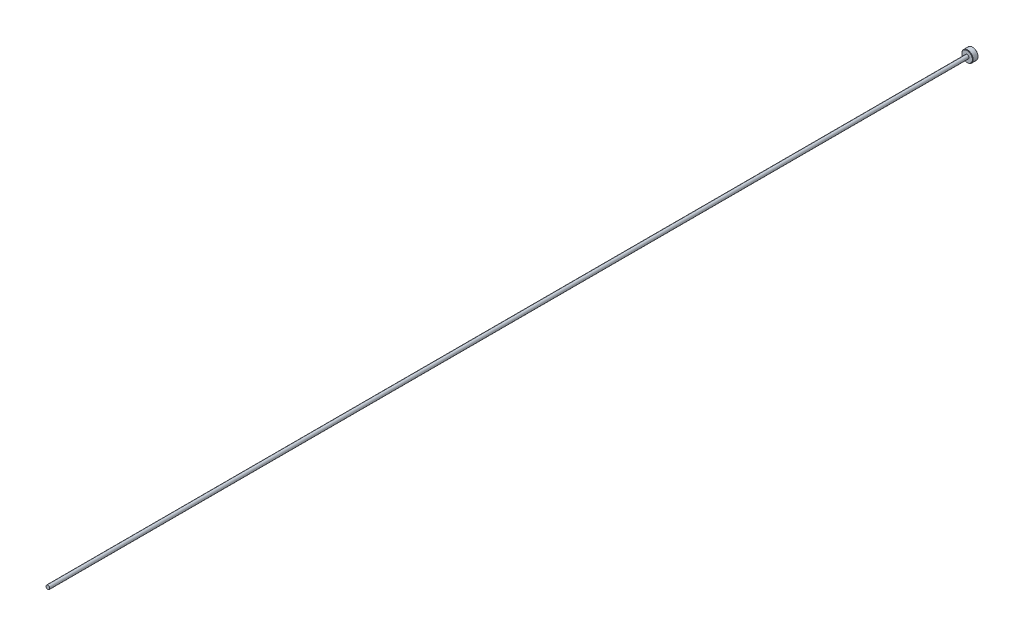
SolidWorks part; units mm, degrees
ref_plane "Front Plane" through (0, 0, 0) normal (0, 0, 1) x (1, 0, 0)
ref_plane "Top Plane" through (0, 0, 0) normal (0, 1, 0) x (1, 0, 0)
ref_plane "Right Plane" through (0, 0, 0) normal (1, 0, 0) x (0, 0, -1)
other "Configuration Table"
sketch "Sketch1" plane through (0, 0, 0) normal (0, 0, 1) x (1, 0, 0)
  circle A0 centre (0, 0) radius 1
  dimension "D1" = 2
extrude "Boss-Extrude1" add sketch "Sketch1" along normal blind 490
sketch "Sketch2" plane through (0, 0, 0) normal (0, 0, -1) x (-1, 0, 0)
  circle A0 centre (0, 0) radius 3
  dimension "D1" = 6
extrude "Boss-Extrude2" add sketch "Sketch2" along normal blind 3
chamfer "Chamfer1" distance 0.2 angle 45 2 edges at (-3, 0, 0) (-3, 0, -3)
